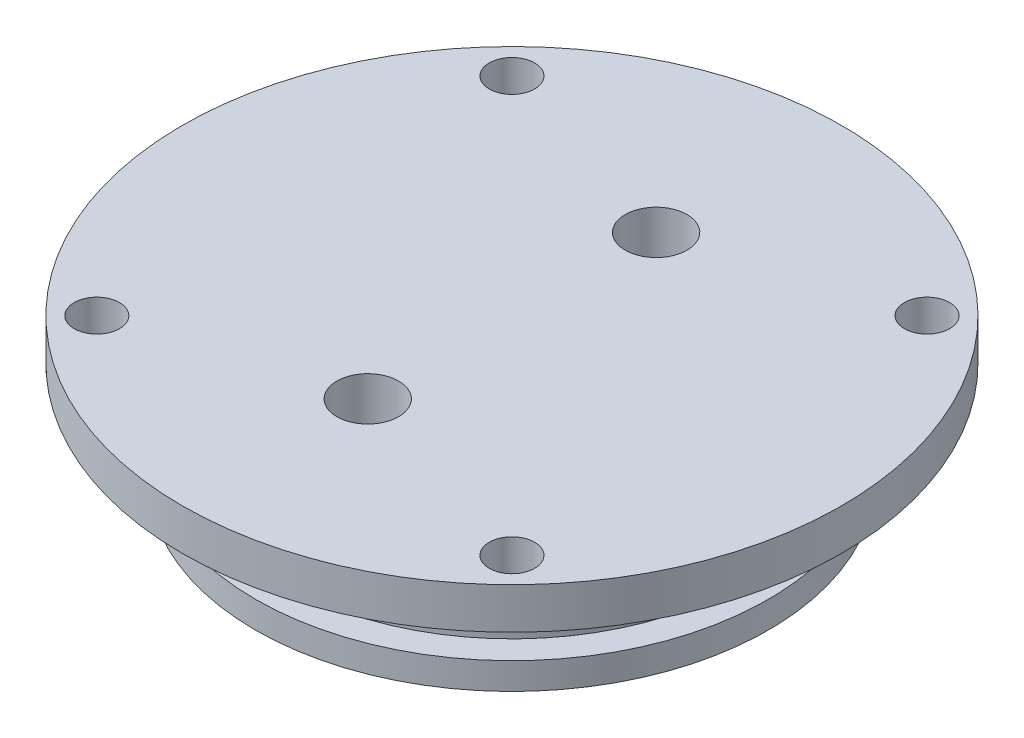
from build123d import *

# Parameters (mm, degrees)
MM_1_D              = 2.2
MM_1_DEPTH          = 7.1
MM_1_TIP            = 0.660946681
SKETCH_7_R          = 2.5
SKETCH_7_R_2        = 1.5
CUT_EXTRUDE_1_DEPTH = 5
SKETCH_8_R          = 1.5
CUT_EXTRUDE_2_DEPTH = 5


with BuildPart() as part:
    # 草图1 → 旋转1 (revolve)
    with BuildSketch(Plane.XY, mode=Mode.PRIVATE) as revolve_1_sk:
        Polygon((0, 0), (12.45, 0), (12.45, 1.295), (11.1546, 1.295), (11.1546, 3.708), (12.45, 3.708), (12.45, 5), (16, 5), (16, 7), (0, 7), align=None)
    revolve(revolve_1_sk.sketch.rotate(Axis((0, 7, 0), (0, -1, 0)), 90), axis=Axis((0, 7, 0), (0, -1, 0)))

    # 大小mm 暗销孔1
    with Locations(Plane(origin=(0, 7, 0), x_dir=(1, 0, 0), z_dir=(0, 1, 0))):
        with Locations((-10.076271632, -10.076271632), (-10.076271632, 10.076271632), (10.076271632, 10.076271632), (10.076271632, -10.076271632)):
            Hole(MM_1_D / 2, depth=MM_1_DEPTH)
            with Locations((0, 0, -(MM_1_DEPTH + MM_1_TIP / 2))):  # 118° drill point
                Cone(0, MM_1_D / 2, MM_1_TIP, mode=Mode.SUBTRACT)

    # 草图7 → 切除-拉伸1 (cut)
    with BuildSketch(Plane.XZ):
        with Locations(Location((-9, 0, 0), (0, 0, 270))):
            Circle(SKETCH_7_R)
        with Locations(Location((9, 0, 0), (0, 0, 270))):
            Circle(SKETCH_7_R)
        with Locations(Location((0, -7, 0), (0, 0, 270))):
            Circle(SKETCH_7_R_2)
        with Locations(Location((0, 7, 0), (0, 0, 270))):
            Circle(SKETCH_7_R_2)
    extrude(amount=-CUT_EXTRUDE_1_DEPTH, mode=Mode.SUBTRACT)

    # 草图8 → 切除-拉伸2 (cut)
    with BuildSketch(Plane.XZ.offset(-5)):
        with Locations(Location((0, 7, 0), (0, 0, 270))):
            Circle(SKETCH_8_R)
        with Locations(Location((0, -7, 0), (0, 0, 270))):
            Circle(SKETCH_8_R)
    extrude(amount=-CUT_EXTRUDE_2_DEPTH, mode=Mode.SUBTRACT)


solid = part.part
